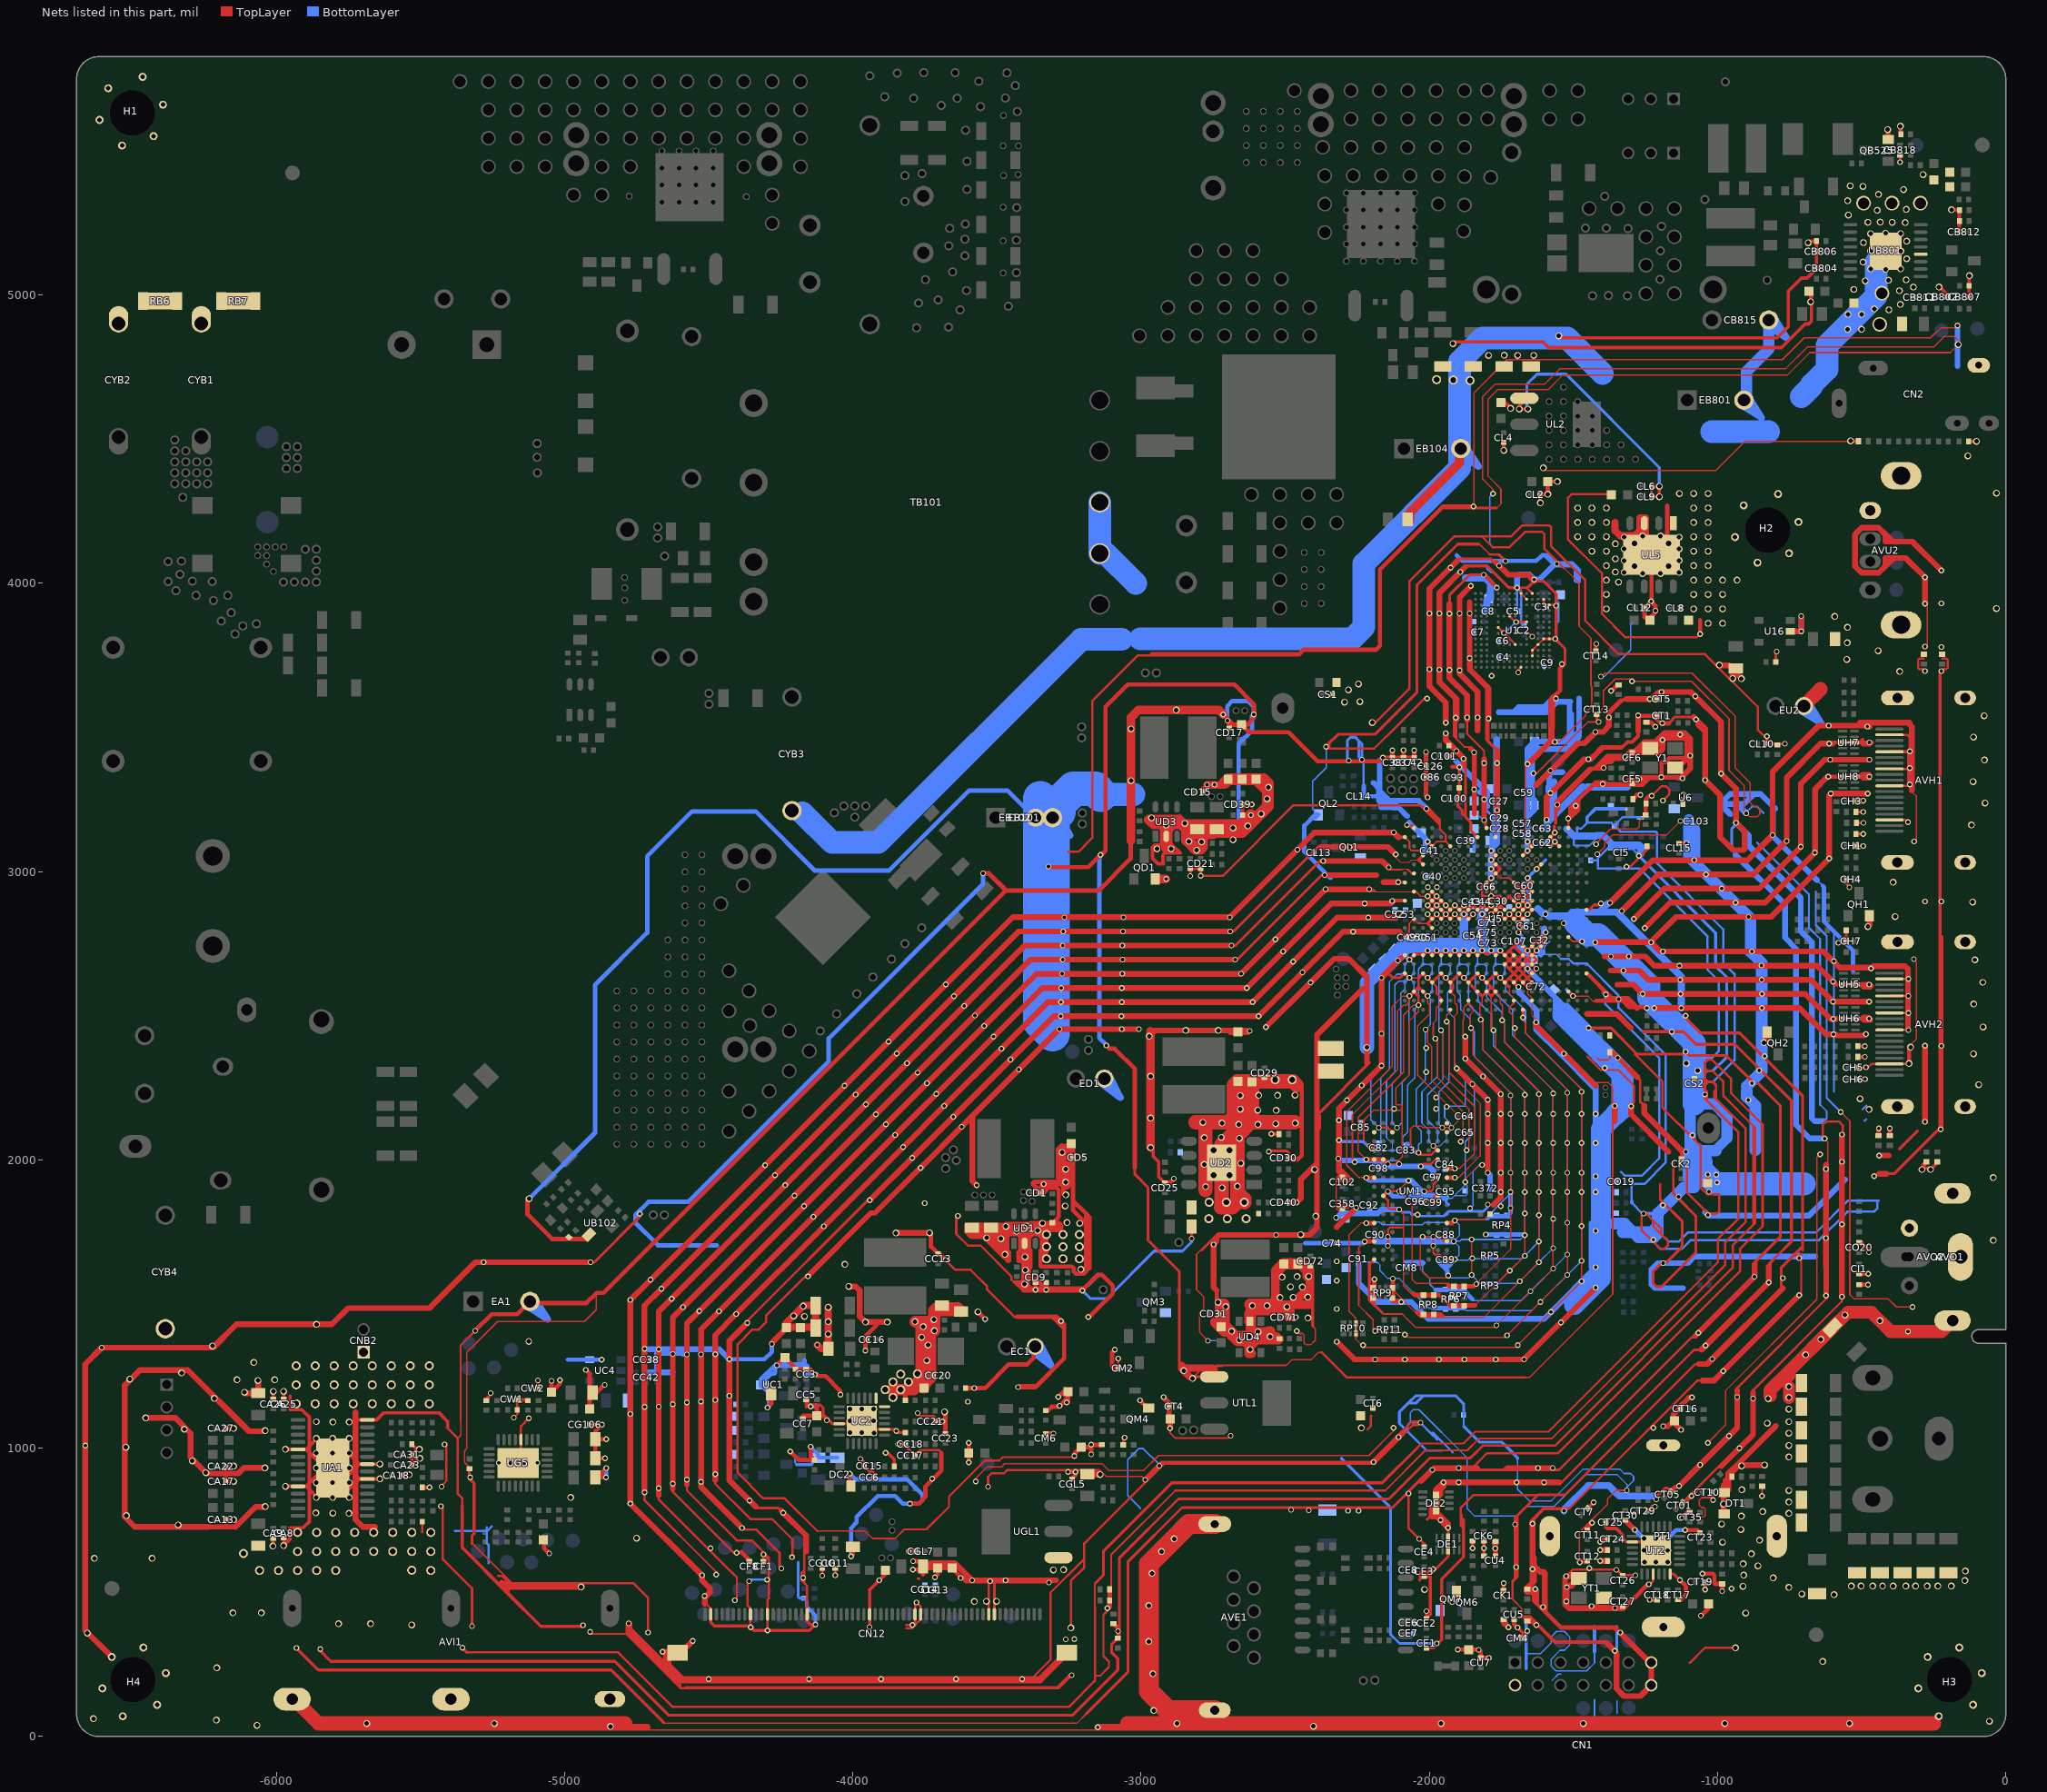
[diagram p0: the nets of this part, all layers, seen from the top]
# Altium PCB MISC84395.PcbDoc (part 15 of 26)
Units mil, origin at the board's own origin, x right, y up, seen from the top; angles counter-clockwise.
Board outline 6692.91 x 5826.77 mil, 2 copper layers (TopLayer, BottomLayer), stack 61.855 mil thick; 951 components, 565 nets, 4374 pads, 1804 vias.
Unrouted connection lines stored in the file: 1.

## Via types
v1: diameter 19.68, hole 11.81, TopLayer to BottomLayer, tented both sides, 1262 vias
v2: diameter 23.62, hole 15.75, TopLayer to BottomLayer, tented both sides, 524 vias
v3: diameter 31.5, hole 19.68, TopLayer to BottomLayer, tented both sides, 11 vias
v4: diameter 24, hole 16, TopLayer to BottomLayer, tented both sides, 6 vias
v5: diameter 19, hole 11.81, TopLayer to BottomLayer, tented both sides, 1 vias

## Nets (pads, with @x,y where several pads share a name; then routed paths per layer and width w, separated by ;. In a path a pad name is that pad's centre, name@x,y a point inside that pad or via, vN(x,y) a via of type N, cw(c..) or ccw(c..) an arc to the next point about the centre after c; other vN are vias at no path point) (continued)
GND: (continued)
  TopLayer w10: v1(-5930,307) -5854,231 -4838,231 -4655.5,48.5 ; v1@-5850,300 -5811,261 -4825.57,261 -4638.07,73.5 -3238.71,73.5 -3081,231.21 -3081,270 -3101.83,290.83 -3101.83,320.27 -3081.36,340.73 DI1.A@-3081,340.73 ; v1(-5354,308) -5337,291 ; RG3.1@-5330,929.27 -5330,894 -5314.1,878.1 -5314.1,703.32 -5321.04,696.38 -5321.04,669.04 ; RG4.1@-5271,1165.73 -5271,1171 -5256,1186 v1(-5256,1191) ; v1(-4910,1645) -4896.88,1645 -4739,1802.88 v1(-4739,1813) ; v1(-4365.93,1434.91) -4365.93,1441.98 v1@-3942.81,1865.09 ; -4331.88,792.13 -4257.32,792.13 v1@-4247.09,781.91 ; v1@-4261.22,1289.7 -4234.62,1316.3 CC11.2@-4234.62,1317 ; v1@-4260.72,1290.2 -4260.42,1290.2 -4236.62,1314 CC11.2@-4233.62,1317 ; -4162,1143 -4155.59,1149.41 -4112.41,1149.41 -4103,1140 -4103,1117.79 -4070.29,1085.08 UC2.4@-4047.48,1085.08 UC2.25@-3978.58,1085.08 ; v1(-3974,963) -3971,963 -3959.73,951.73 CC15.1@-3959.73,938 -3939.89,918.16 -3930.94,918.16 -3926.43,913.64 CC6.1@-3926.43,899 ; UC2.25@-3939.21,1065.39 UC2.14@-3890,1065.39 -3854.39,1065.39 v1(-3849,1060) -3843,1054 RC12.1@-3817.73,1054 ; v1(-3843,1014) CC18.1@-3817.73,1014 ; CC21.2@-3714.26,1093 v1(-3689,1093) ; -3640.73,1743.88 -3640.73,1801.32 v1(-3635.89,1806.16) ; -3638.23,1794.77 v1@-3627.31,1805.69 ; CD4.2@-3586.86,1764.86 CD4.2@-3571.03,1764.86 ; v2@-3535.62,1726.38 -3535.62,1726.88 v2(-3535.62,1729.44) ; -3190,79.79 -3045,224.79 -3045,607 -2858,794 -2128.07,794 -2023.54,898.54 ; -3158.95,531.25 -3131,559.2 -3131,580 ; -3131,571 -3131,580 ; v1(-3080,365.5) -3080,341.73 DI1.A@-3081,340.73 ; -3048,45.5 -3045,48.5 ; -3021.5,1972 -3021.5,1949.44 -2976,1903.94 -2976,1721.14 -2867,1612.14 -2867,1273 -2841.55,1247.55 -2830.55,1247.55 UTL1.1@-2746.27,1247.55 ; v1(-2824.94,1726.94) CD23.1@-2824.94,1769 ; v1(-2691,2792.5) -2678.92,2792.5 -2385.82,3085.6 ; v1(-2686,2743.5) -2672.77,2743.5 -2379.67,3036.6 v1(-2369,3036.6) ; v1(-2673.69,2694.5) -2666.61,2694.5 -2373.51,2987.6 v1(-2363,2987.6) ; v1(-2557,2029) -2555,2031 -2494,2031 -2488.26,2025.26 CD30.2@-2488.26,2006 ; CD71.1@-2488,1454.26 v1(-2463,1454.26) ; CD72.1@-2413,1632.37 -2413,1607.26 -2405,1599.26 -2405,1424 ; -2380.07,2108.87 -2380.07,2153.13 ; -2380.07,2164.9 -2207.65,2337.32 ; v1(-2358.03,3432.68) -2348,3442.71 ; -2348,3427.84 -2348,3442.71 ; -2147.49,2651.47 -2127.88,2631.85 -2100.18,2631.85 U5.E21@-2084.93,2647.11 v1(-2069.18,2631.36) ; v1@-2107.7,2962.07 U5.R21@-2084.93,2962.07 ; -2100.68,2698.28 U5.G21@-2088.87,2710.1 ; v1@-2078.58,3161.48 -2075.1,3158 -2060.39,3158 U5.AA20@-2053.43,3151.04 ; -2043.04,1000.62 -2163.66,880 -2893.62,880 -3131,642.62 -3131,580 ; -2037.68,2631.36 -2025.24,2643.8 U5.E19@-2021.94,2647.11 ; -2034.19,542.19 -2032.41,543.97 -2032.41,570.3 -2031.99,569.88 -2004.02,569.88 -1998.16,575.74 -1998.16,586.5 ; U5.U19@-2021.94,3025.06 -2037.68,3040.81 U5.V19@-2021.94,3056.56 ; CE3.1@-2018,555.27 -2003.67,555.27 -1996.5,562.44 ; CE1.1@-2010.1,306.99 -1987.01,306.99 v1@-1971,323 ; v1@-2010,434.41 v1(-2010,435) -2010.1,434.9 CE2.1@-2010.1,409.44 -1996.5,423.04 -1996.5,562.44 ; -2008.15,753.2 -1997.51,763.84 -1997.51,799.39 -1983.5,813.41 -1983.5,856.57 -1958.07,882 v1(-1951,882) ; v1(-2006.19,2851.83) U5.L18@-1990.44,2836.08 ; v1(-2006.19,3103.32) -2005.7,3103.32 U5.W18@-1990.44,3088.05 ; v1@-2005.7,2945.84 v1(-2005.7,2946.32) ; U5.K18@-1990.44,2804.59 -2006.19,2820.34 U5.L18@-1990.44,2836.08 ; v1(-1975,323) v1@-1971,323 ; v1@-1974.75,2946.26 v1(-1974.26,2946.26) ; v1@-1974.51,2883.14 U5.M17@-1958.94,2867.58 v1(-1943.2,2851.83) ; -1935,734 v1(-1935,724) -1935,623.94 -1996.5,562.44 ; -1930.21,3928.74 -1930.21,3958.86 -1859.64,4029.43 v1(-1811.34,4029.43) ; U5.C16@-1927.45,2584.12 -1919.58,2591.99 -1919.58,2607.73 ; -1903,4078 -1896.15,4084.84 -1789.01,4084.84 -1775.17,4071 -1768.09,4071 ; C100.1@-1901.14,3256 -1901.14,3225.95 -1885.32,3210.13 -1885.32,3200.23 -1874.66,3189.57 ; C93.1@-1896.55,3326.48 -1896.55,3361.45 v1(-1896,3362) ; v1@-1896.54,3360.92 C100.1@-1896.54,3253 -1874.66,3253 ; -1889.81,769 -1889.81,731.81 -1881.5,723.5 ; -1881.5,753.5 -1881.5,723.5 ; v1(-1881.48,3390.91) -1874.66,3384.08 -1874.66,3189.57 ; -1876.65,4054.84 -1871.65,4059.84 -1799.36,4059.84 -1723.74,3984.21 v1@-1695.12,3984.21 ; -1874.66,3218 -1874.66,3189.57 ; -1872.04,3186.96 -1856.54,3171.45 ; v1(-1848.71,2851.83) U5.L14@-1864.46,2836.08 v1(-1880.2,2851.83) ; -1834.29,989.29 -1857.58,966 -1998.5,966 -2140.5,824 -2870.43,824 -3075,619.43 -3075,346.73 DI1.A@-3081,340.73 ; U5.Y13@-1832.96,3119.55 -1856.54,3143.13 -1856.54,3171.45 ; -1829.83,4136 -1901.56,4136 -2042.88,3994.68 -2042.88,3622.54 -2189.58,3475.84 -2317.22,3475.84 -2348,3445.06 -2348,3442.71 ; v1(-1817.21,2851.83) U5.L12@-1801.46,2836.08 v1(-1785.72,2851.83) -1754.22,2883.33 ; -1817.21,2946.32 U5.R12@-1801.46,2962.07 U5.T11@-1769.97,2993.56 ; -1815.86,2881.97 U5.M12@-1801.46,2867.58 ; -1815.86,2884.68 U5.M13@-1832.96,2867.58 -1848.71,2883.33 U5.M14@-1864.46,2867.58 ; v1@-1804.97,3174.59 -1804.97,3154.55 U5.AA12@-1801.46,3151.04 ; -1802.21,3642.82 -1802.21,3458.12 -1796.36,3452.27 ; U5.M12@-1801.46,2870.29 U5.M12@-1801.46,2867.58 ; -1796.36,3457.12 -1796.36,3452.27 ; v1(-1785.72,3072.3) U5.V11@-1769.97,3056.56 v1(-1785.72,3040.81) U5.U11@-1769.97,3025.06 ; -1764.97,3420.88 -1796.36,3452.27 ; -1757.16,4098.16 v1(-1736,4077) v1@-1741,4077 ; -1754.22,2914.82 U5.N10@-1738.47,2899.08 ; CL3.2@-1752,4626.81 -1738.35,4626.81 v2(-1718.44,4606.9) ; U5.M10@-1738.47,2867.58 -1754.22,2883.33 ; -1722.72,2599.86 U5.D10@-1738.47,2615.61 ; -1722.49,2663.09 U5.F9@-1706.98,2678.6 ; -1710.17,539.65 -1703.17,546.65 ; U5.D9@-1706.98,2616.08 -1691.46,2631.59 ; U5.R9@-1706.98,2962.07 U5.P8@-1675.48,2930.57 ; v1@-1701.78,3865.84 v1@-1701.54,3866.08 ; -1699.81,568.49 -1699.81,617.11 -1694.5,622.42 ; -1692.46,2664.08 U5.F9@-1706.98,2678.6 ; v1(-1691.23,2599.86) U5.D9@-1706.98,2615.61 -1722.72,2631.36 ; v1(-1691.23,2788.84) U5.K8@-1675.48,2804.59 v1(-1691.23,2820.34) ; v1(-1675.48,2493.56) -1675.48,2495.03 U5.A8@-1675.48,2521.12 ; U5.M8@-1675.48,2867.58 v1(-1691.23,2883.33) ; U5.V8@-1675.48,3056.56 v1(-1659.73,3072.3) U5.W7@-1643.98,3088.05 v1(-1659.73,3103.8) ; DU5.A@-1665.83,510 -1660.83,515 -1642.19,533.64 -1642.19,568.49 ; -1662.67,3984.21 -1659.9,3984.21 -1636.37,4007.74 -1604.65,4007.74 -1560.26,3963.35 v1(-1560.26,3922.09) v1@-1560.26,3806.02 ; v1(-1659.73,2851.83) U5.L8@-1675.48,2836.08 ; v1(-1659.73,2977.82) U5.R7@-1643.98,2962.07 -1659.73,2946.32 ; v1@-1657.98,2853.58 U5.M7@-1643.98,2867.58 v1(-1659.73,2883.33) ; v1@-1628.47,2662.62 U5.E7@-1643.98,2647.11 ; v1(-1628.47,2663.09) U5.F7@-1643.98,2678.6 U5.F7@-1644.22,2678.84 ; v1(-1628.24,3009.31) U5.U6@-1612.49,3025.06 ; -1598.24,3253.76 -1593.24,3258.76 ; v1(-1596.74,2788.84) U5.J6@-1612.49,2773.09 ; U5.W5@-1580.99,3088.05 v1(-1565.24,3103.8) ; -1566.58,3158.12 -1566.58,3136.64 v1(-1565.24,3135.3) U5.Y5@-1580.99,3119.55 v1(-1565.24,3103.8) ; -1561.65,3168 -1561.65,3206.68 ; v1@-1561.43,3804.84 -1529.21,3772.62 -1529.21,3722.18 v1@-1531.71,3719.68 ; v1@-1553.82,3235.84 ccw(c-1565.89,3247.91) v1@-1553.32,3236.36 ; -1553.32,3243.41 v1@-1553.32,3236.36 ; -1553.15,3219.17 -1552.37,3219.17 -1550.77,3217.56 -1561.65,3206.68 ; U5.W4@-1549.5,3088.05 v1(-1565.24,3103.8) ; -1548.82,3247.91 cw(c-1565.89,3247.91) -1549.29,3243.9 cw(c-1565.89,3247.91) -1553.15,3236.55 cw(c-1565.89,3247.91) v1@-1553.32,3236.36 ; -1547.84,3252.42 -1556.65,3243.61 -1561.65,3238.61 v1@-1561.65,3228.01 ; -1532.05,838 -1622.92,838 -1623.92,837 -1703.17,757.75 ; v1(-1524.71,468.43) -1524.71,461.58 -1518.87,455.74 ; YT1.2@-1492.8,548.46 -1518.87,522.4 -1518.87,455.74 ; U5.M1@-1455.01,2867.58 -1445.68,2867.58 -1428.68,2884.58 -1409.61,2884.58 v1(-1404.77,2889.43) ; v1(-1447.69,2457.53) -1370.06,2457.53 -1279.5,2366.97 -1118.51,2366.97 v1(-1110.96,2374.52) -1109.81,2374.52 -1097.21,2361.92 -969.93,2361.92 -881,2273 v1(-881,2266) ; v1(-1437.03,452.26) -1423.97,452.26 ; CT13.1@-1419.65,3545.01 -1419.65,3525.74 v1(-1412.65,3518.74) v1@-1412.65,3524.18 ; YT1.4@-1394.69,481.54 -1423.97,452.26 ; v1(-1377.21,3534.74) -1377.21,3545.75 -1324.96,3598 -1317,3598 ; v1@-1351.29,576.23 -1347.79,576.23 CT26.1@-1330.28,558.73 ; -1329.48,687.49 -1317,675 UT2.14@-1295.78,675 UT2.25@-1243.42,675 ; CT26.1@-1329.01,559 CT26.1@-1329.28,558.73 -1285.27,558.73 v1(-1285,559) ; -1301.24,2454.76 -1301.24,2458.01 -1301.24,2463.17 ; -1291.17,475.17 -1238.47,527.88 v1(-1238.47,528.06) -1235.68,528.06 -1223.73,540 UT2.21@-1223.73,563.58 ; v1@-1267.75,3053.91 -1244.91,3076.75 RI5.1@-1244.91,3087.74 ; -1258.38,2444.97 -1157.03,2444.97 -1127.97,2444.97 ; v1(-1213.06,822.88) -1213.06,831.53 -1182.6,862 -1173.34,862 CT05.1@-1162.17,850.83 ; -1197.84,1860.95 -1122.5,1785.61 -1122.5,1698.91 -1178.29,1643.12 v1@-1193.88,1643.12 ; v1(-1189,1641.8) -1195.2,1641.8 -1223.84,1613.16 -1223.84,1571.78 -1212.22,1560.16 -1194.78,1560.16 -1075.5,1679.44 -1075.5,1805.07 v1@-1135.34,1864.92 ; -1171.65,3464.32 -1169.93,3466.04 -1112.67,3466.04 -1095.15,3448.52 -1091.26,3444.63 -1091.96,3444.63 -1095.15,3441.45 ; -1168.83,3514 -1155.59,3527.24 -1155.59,3529.98 -1149.73,3535.84 -1083.2,3535.84 -1075.68,3535.84 v1@-1067.83,3528 ; UT2.24@-1164.68,563.58 -1151.58,563.58 v1(-1131,543) ; -1150.84,1880.42 v1@-1135.34,1864.92 ; v1(-1135.34,1871.76) v1@-1135.34,1864.92 ; -1127,2444 -1127.97,2444.97 ; v1(-1111,2500) -1111,2491.71 -1059.21,2439.92 -923.92,2439.92 -705,2221 -705,1700.49 ; CT10.1@-1022.43,847 -1022.43,825.57 v1@-1019.43,822.57 ; CT10.1@-1019.43,847 v1@-1019.43,822.57 ; v1(-1016,820) -1016.85,820 v1@-1019.43,822.57 ; v1@-881.16,1593.06 -877.5,1596.72 -877.5,1638.3 -867,1648.8 ; -867,1610 -867,1648.8 ; -860.53,2266.23 -783,2188.69 -783,1732.8 -842.9,1672.9 ; v1(-856.07,2310.07) v1@-849.22,2310.07 ; -852.9,1662.9 -842.9,1672.9 ; -828,1603 -828,1632.64 -818,1642.64 ; -818,1603 -818,1642.64 ; -813.82,1646.82 -799.82,1660.82 ; RU10.1@-798.27,3727 -798.27,3761.73 -797,3763 v1(-795,3763) ; -792.7,1535.7 -779,1549.41 -779,1626.49 -778.5,1626.99 -737.4,1668.09 -705,1700.49 ; v1@-716.84,1668.09 -712,1672.94 ; v1@-712,1658.36 v1@-712,1663.25 ; -705,1685.94 -705,1700.49 ; v1(-582,2753) -576.84,2758.16 CH7.1@-554.1,2758.16 DH4.A@-554.1,2796.16 ; CH4.1@-553.57,2973 -553.57,2957.73 -542.83,2947 v1(-542.83,2945) ; DH1.A@-519.91,3206.79 v1(-494.88,3206.79) ; CH1.2@-519.64,3088.99 -495.07,3088.99 v1(-494.88,3088.79) ; DH3.A@-519.64,3130.29 v1(-494.88,3130.29) ; DH2.A@-519.14,3168.79 v1(-494.38,3168.79) ; CH5.2@-513.63,2319.88 -486.37,2319.87 v1(-485.37,2320.87) ; v1@-473.04,3502.79 -464.65,3511.18 -353.48,3511.18 ; -414.73,1952 -387.4,1952 v1@-228.83,2110.57 ; AVH1.5@-403.84,3415.35 v1@-335.04,3415.32 ; -370,2037.18 -307.18,2100 ; v1@-367,5460 CB818.1@-367,5485.54 ; v1@-334.05,3301.12 v1(-333.38,3301.79) ; v1@-333.38,3415.65 -333.38,3465.16 ; v1(-223.83,2395) -221.74,2397.09 -221.74,2774 ; v1(-223.83,3695.57) -228.83,3690.57 v1@-228.83,2110.57 ; v1@-221.74,2394.26 -221.74,2110.82 v1(-226.58,2105.97) -228.83,2108.23 v1@-228.83,2110.57 ; U5.G21@-2088.87,2710.1 U5.G21@-2084.93,2710.1 ; U5.G21@-2088.87,2710.1 U5.G21@-2084.93,2710.1 ; U5.G21@-2084.93,2710.1 v1(-2069.18,2694.35) U5.G20@-2053.43,2710.1 -2049.34,2714.2 -2026.03,2714.2 U5.G19@-2021.94,2710.1 ; U5.C20@-2053.43,2584.12 v1(-2069.18,2568.36) U5.C20@-2053.43,2584.12 ; U5.C20@-2053.43,2584.12 -2037.69,2599.86 ; U5.C20@-2053.43,2584.12 -2037.69,2599.86 ; U5.C20@-2053.43,2584.12 -2037.69,2568.36 U5.C20@-2053.43,2584.12 ; -2037.69,2599.86 U5.C19@-2021.94,2584.12 ; -2037.69,2599.86 U5.C19@-2021.94,2584.12 ; -2037.69,2599.86 v1(-2006.19,2568.36) U5.C19@-2021.94,2584.12 ; U5.E19@-2021.94,2647.11 v1(-2006.19,2631.36) ; U5.E19@-2021.94,2647.11 v1(-2006.19,2631.36) ; U5.E19@-2021.94,2647.11 v1(-2006.19,2631.36) ; U5.G19@-2021.94,2710.1 v1(-2006.19,2725.84) ; U5.G19@-2021.94,2710.1 v1(-2006.19,2725.84) ; v1(-2006.19,2631.36) v1@-2005.71,2630.88 ; v1(-2006.19,2631.36) U5.D18@-1990.44,2615.61 ; v1(-2006.19,2631.36) v1@-2005.71,2630.88 ; v1(-2006.19,2725.84) U5.G18@-1990.44,2710.1 ; v1(-2006.19,2725.84) U5.G18@-1990.44,2710.1 ; v1@-2005.71,2630.88 U5.D18@-1990.44,2615.61 ; v1@-2005.71,2630.88 U5.D18@-1990.44,2615.61 ; U5.D18@-1990.44,2615.61 U5.E17@-1958.94,2647.11 ; U5.D18@-1990.44,2615.61 U5.E17@-1958.94,2647.11 ; U5.G18@-1990.44,2710.1 v1(-1974.69,2725.84) ; U5.G18@-1990.44,2710.1 v1(-1974.69,2725.84) ; U5.L18@-1990.44,2836.08 v1(-1974.69,2851.83) U5.L17@-1958.94,2836.08 v1(-1943.2,2851.83) ; U5.N18@-1990.44,2899.08 v1(-1974.69,2883.33) ; U5.N18@-1990.44,2899.08 v1(-2006.19,2883.33) U5.M18@-1990.44,2867.58 v1(-1974.69,2883.33) ; U5.N18@-1990.44,2899.08 v1(-2006.19,2914.82) U5.P18@-1990.44,2930.57 v1(-1974.69,2914.82) ; U5.N18@-1990.44,2899.08 v1(-1974.69,2914.82) ; v1(-1974.69,2725.84) U5.G17@-1958.94,2710.1 v1(-1943.2,2725.84) U5.G16@-1927.45,2710.1 ; v1(-1974.69,2883.33) U5.N17@-1958.94,2899.08 ; v1(-1974.69,2914.82) U5.N17@-1958.94,2899.08 ; v1@-1971,323 -1957.5,336.5 -1957.5,546.28 -1881.5,622.29 -1881.5,723.5 ; U5.E17@-1958.94,2647.11 v1(-1943.2,2631.36) ; U5.E17@-1958.94,2647.11 v1(-1943.2,2631.36) ; U5.N17@-1958.94,2899.08 v1(-1943.2,2883.33) U5.M16@-1927.45,2867.58 ; v1(-1943.2,2631.36) U5.D16@-1927.45,2615.61 ; v1(-1943.2,2631.36) U5.D16@-1927.45,2615.61 ; v1(-1943.2,2851.83) U5.M16@-1927.45,2867.58 ; v1(-1943.2,2851.83) U5.L16@-1927.45,2836.08 v1(-1911.7,2851.83) U5.L15@-1895.95,2836.08 v1(-1880.2,2851.83) ; U5.D16@-1927.45,2615.61 U5.E15@-1895.95,2647.11 ; U5.D16@-1927.45,2615.61 -1920.77,2622.29 ; U5.D16@-1927.45,2615.61 -1920.77,2622.29 ; U5.D16@-1927.45,2615.61 -1919.58,2607.73 ; U5.D16@-1927.45,2615.61 -1919.58,2607.73 ; U5.G16@-1927.45,2710.1 v1(-1911.7,2725.84) ; U5.G16@-1927.45,2710.1 v1(-1911.7,2725.84) ; U5.M16@-1927.45,2867.58 v1(-1911.7,2883.33) U5.M15@-1895.95,2867.58 ; -1920.77,2622.29 U5.E15@-1895.95,2647.11 ; v1(-1911.7,2725.84) -1895.95,2710.1 v1(-1880.21,2725.84) ; U5.E15@-1895.95,2647.11 v1(-1880.21,2631.36) ; U5.E15@-1895.95,2647.11 v1(-1880.21,2631.36) ; U5.M15@-1895.95,2867.58 v1(-1880.2,2851.83) ; U5.M15@-1895.95,2867.58 v1(-1880.2,2883.33) U5.M14@-1864.46,2867.58 ; v1(-1880.21,2631.36) U5.D14@-1864.46,2615.61 ; v1(-1880.21,2725.84) U5.G14@-1864.46,2710.1 ; v1(-1880.21,2725.84) U5.G14@-1864.46,2710.1 ; v1(-1880.2,2851.83) U5.M14@-1864.46,2867.58 ; -1874.66,3189.57 -1856.54,3171.45 ; U5.D14@-1864.46,2615.61 U5.C13@-1832.96,2584.12 ; U5.D14@-1864.46,2615.61 U5.E13@-1832.96,2647.11 v1(-1817.21,2631.36) U5.D12@-1801.46,2615.61 ; U5.G14@-1864.46,2710.1 v1(-1848.71,2725.84) ; U5.G14@-1864.46,2710.1 v1(-1848.71,2725.84) ; v1(-1848.71,2725.84) U5.G13@-1832.96,2710.1 ; v1(-1848.71,2725.84) U5.G13@-1832.96,2710.1 ; U5.C13@-1832.96,2584.12 -1817.21,2568.36 ; U5.C13@-1832.96,2584.12 -1817.21,2568.36 ; U5.G13@-1832.96,2710.1 v1(-1817.21,2725.84) ; U5.G13@-1832.96,2710.1 v1(-1817.21,2725.84) ; -1817.21,2568.36 U5.C12@-1801.46,2584.12 ; -1817.21,2568.36 U5.C12@-1801.46,2584.12 ; v1(-1817.21,2725.84) -1805.4,2714.04 -1797.52,2714.04 v1(-1785.72,2725.84) ; U5.C12@-1801.46,2584.12 -1785.72,2568.36 ; U5.C12@-1801.46,2584.12 -1785.72,2599.86 ; U5.D12@-1801.46,2615.61 -1785.72,2599.86 ; U5.D12@-1801.46,2615.61 -1785.72,2599.86 ; U5.D12@-1801.46,2615.61 -1781.31,2635.77 ; U5.D12@-1801.46,2615.61 -1781.31,2635.77 ; U5.D12@-1801.46,2615.61 U5.E11@-1769.97,2647.11 ; U5.M12@-1801.46,2867.58 v1(-1785.72,2883.33) U5.M11@-1769.97,2867.58 v1(-1754.22,2851.83) U5.L10@-1738.47,2836.08 v1(-1722.72,2851.83) ; -1785.72,2568.36 U5.C11@-1769.97,2584.12 ; -1785.72,2568.36 U5.C11@-1769.97,2584.12 ; -1785.72,2599.86 U5.C11@-1769.97,2584.12 ; -1785.72,2599.86 U5.C11@-1769.97,2584.12 ; v1(-1785.72,2725.84) U5.G11@-1769.97,2710.1 ; v1(-1785.72,2725.84) U5.G11@-1769.97,2710.1 ; -1781.31,2635.77 U5.E11@-1769.97,2647.11 ; -1781.31,2635.77 U5.E11@-1769.97,2647.11 ; U5.E11@-1769.97,2647.11 v1(-1754.22,2631.36) ; U5.E11@-1769.97,2647.11 v1(-1754.22,2631.36) ; U5.G11@-1769.97,2710.1 v1(-1754.22,2725.85) ; U5.G11@-1769.97,2710.1 v1(-1754.22,2725.85) ; U5.T11@-1769.97,2993.56 v1(-1785.72,3009.31) U5.U11@-1769.97,3025.06 ; U5.T11@-1769.97,2993.56 -1754.22,3009.31 U5.U11@-1769.97,3025.06 ; v1(-1754.22,2631.36) U5.D10@-1738.47,2615.61 ; v1(-1754.22,2725.85) U5.G10@-1738.47,2710.1 ; -1754.22,2883.33 U5.N10@-1738.47,2899.08 ; U5.D10@-1738.47,2615.61 -1722.72,2631.36 ; U5.G10@-1738.47,2710.1 -1722.72,2694.35 ; U5.G10@-1738.47,2710.1 -1722.72,2725.85 ; U5.N10@-1738.47,2899.08 -1722.72,2914.82 U5.N9@-1706.98,2899.08 ; -1722.72,2631.36 -1706.98,2647.11 ; -1722.72,2694.35 U5.F9@-1706.98,2678.6 ; -1722.72,2694.35 U5.G9@-1706.98,2710.1 ; -1722.72,2694.35 U5.F10@-1738.47,2678.6 -1706.98,2647.11 ; -1722.72,2725.85 U5.G9@-1706.98,2710.1 ; -1722.72,2725.85 -1706.98,2741.6 ; v1(-1722.72,2851.83) U5.L9@-1706.98,2836.08 ; v1(-1722.72,2851.83) v1(-1691.23,2883.33) ; -1706.98,2647.11 -1691.23,2662.86 ; -1706.98,2647.11 -1691.46,2631.59 ; U5.F9@-1706.98,2678.6 -1691.23,2694.35 ; U5.G9@-1706.98,2710.1 -1691.23,2694.35 ; -1706.98,2741.6 -1691.23,2757.34 U5.H8@-1675.48,2741.6 v1(-1659.73,2725.85) ; -1706.98,2741.6 U5.G8@-1675.48,2710.1 ; U5.L9@-1706.98,2836.08 v1(-1691.23,2851.83) ; U5.L9@-1706.98,2836.08 v1(-1691.23,2820.34) ; U5.N9@-1706.98,2899.08 v1(-1691.23,2883.33) ; U5.N9@-1706.98,2899.08 -1691.23,2914.82 ; -1703.17,546.65 v1(-1703.17,736) -1703.17,757.75 ; -1703.17,546.65 -1697.31,552.5 -1694.5,555.31 -1694.5,622.42 ; -1703.17,757.75 -1694.5,766.42 -1694.5,622.42 ; -1691.46,2631.59 -1675.71,2647.34 ; -1691.46,2631.59 U5.D8@-1675.48,2615.61 ; -1691.23,2662.86 U5.F8@-1675.48,2678.6 ; -1691.23,2662.86 -1675.71,2647.34 ; -1691.23,2694.35 U5.G8@-1675.48,2710.1 ; -1691.23,2694.35 U5.F8@-1675.48,2678.6 ; v1(-1691.23,2820.34) U5.L8@-1675.48,2836.08 ; v1(-1691.23,2851.83) U5.L8@-1675.48,2836.08 ; v1(-1691.23,2851.83) v1(-1659.73,2883.33) ; v1(-1691.23,2883.33) U5.N8@-1675.48,2899.08 ; -1691.23,2914.82 U5.P8@-1675.48,2930.57 ; -1691.23,2914.82 U5.N8@-1675.48,2899.08 ; -1675.71,2647.34 -1659.73,2631.36 ; -1675.71,2647.34 v1@-1659.96,2663.09 ; U5.D8@-1675.48,2615.61 -1659.73,2631.36 ; U5.D8@-1675.48,2615.61 -1659.73,2599.86 U5.D7@-1643.98,2615.61 -1659.73,2631.36 ; U5.F8@-1675.48,2678.6 v1@-1659.96,2663.09 ; U5.F8@-1675.48,2678.6 -1659.73,2694.35 ; U5.G8@-1675.48,2710.1 -1659.73,2694.35 ; U5.G8@-1675.48,2710.1 v1(-1659.73,2725.85) ; U5.N8@-1675.48,2899.08 v1(-1659.73,2883.33) ; U5.N8@-1675.48,2899.08 -1659.73,2914.82 ; U5.P8@-1675.48,2930.57 -1659.73,2946.32 ; U5.P8@-1675.48,2930.57 -1659.73,2914.82 ; v1@-1659.96,2663.09 U5.F7@-1644.22,2678.84 ; v1@-1659.96,2663.09 U5.E7@-1643.98,2647.11 ; -1659.73,2631.36 U5.E7@-1643.98,2647.11 ; -1659.73,2694.35 U5.G7@-1643.98,2710.1 ; -1659.73,2694.35 U5.F7@-1644.22,2678.84 ; v1(-1659.73,2725.85) U5.G7@-1643.98,2710.1 ; v1(-1659.73,2725.85) U5.H7@-1643.98,2741.6 ; v1(-1659.73,2883.33) U5.N7@-1643.98,2899.08 -1659.73,2914.82 ; -1659.73,2914.82 U5.P7@-1643.98,2930.57 -1659.73,2946.32 ; U5.F7@-1644.22,2678.84 -1628.47,2694.58 U5.G7@-1643.98,2710.1 ; U5.G7@-1643.98,2710.1 v1(-1628.24,2725.85) ; U5.H7@-1643.98,2741.6 v1(-1628.24,2725.85) ; U5.H7@-1643.98,2741.6 -1628.24,2757.34 ; v1(-1628.24,2725.85) U5.H6@-1612.49,2741.6 ; -1628.24,2757.34 U5.H6@-1612.49,2741.6 ; -1628.24,2757.34 U5.J6@-1612.49,2773.09 ; U5.H6@-1612.49,2741.6 -1596.74,2757.34 U5.J6@-1612.49,2773.09 ; -1561.65,3206.68 v1@-1561.65,3228.01 ; v1@-1561.65,3228.01 -1556.65,3233.01 v1@-1553.32,3236.34 ; -1518.87,455.74 -1513.01,449.88 -1426.35,449.88 -1424.96,451.27 -1423.97,452.26 ; -1127.97,2444.97 -1119.41,2444.97 -1075.37,2400.92 -940.08,2400.92 v1@-849.22,2310.07 ; -867,1648.8 -842.9,1672.9 ; v1@-849.22,2310.07 -744,2204.85 -744,1716.64 -799.82,1660.82 ; -818,1642.64 -799.82,1660.82 ; CL9.1@-1229.64,4300 CL6.1@-1229.64,4336 v2(-1202.37,4336) -1202.37,4304 -1204.37,4302 v2(-1202.37,4300) CL9.1@-1229.64,4300
  TopLayer w11: CN12.2@-4493.03,423.98 -4493.03,396.03 -4480.56,383.56 -4358.56,383.56 -4342.66,367.66 -4150.34,367.66 v1(-4130,388) -4131,389 -4148,389 -4158.38,399.38 CN12.19@-4158.38,423.98 ; v1(-3942,379.59) -3941.85,379.73 CN12.30@-3941.85,423.98 -3941.85,508.15
  TopLayer w11.81: RP10.4@-2254.71,1389.73 RP10.3@-2254.71,1433.03 ; v2(-1918,4831) -1911.91,4837.09 -1606.05,4837.09 -1586.33,4817.38 -778.62,4817.38 -696.53,4899.47 -684.36,4899.47 -674.97,4908.86 -674.97,4996.97 ; v2(-1551,4858) -1544,4851 -794,4851 -755.02,4889.98 -755.02,5012.48 -709.39,5058.11 -689.48,5058.11 -657.46,5090.12 CB804.1@-657.46,5091.94 ; v2(-686,5181) -680.48,5186.52 RB803.1@-657.24,5186.52 ; CB813.1@-683.81,5013 -677,5006.19 v2(-677,4976) v2@-674.97,4973.97 ; CB804.1@-659.89,5091.94 CB804.1@-657.46,5091.94 ; CB804.1@-657.46,5089.94 CB804.1@-657.46,5091.94 ; RB803.1@-657.24,5190.52 -657.24,5092.17 CB804.1@-657.46,5091.94 ; v2(-232.29,5027.24) -229.24,5027.24 -206.27,5004.27 CB802.1@-206.27,4992.32 ; v2(-189,5295) -162.29,5295 RB822.1@-161.42,5294.13 RB812.1@-161.42,5256.13 CB812.1@-161.42,5218 ; CB807.2@-127.54,4992.32 RB827.1@-127.54,5031.32 -127.54,5066.46 v2(-127,5067)